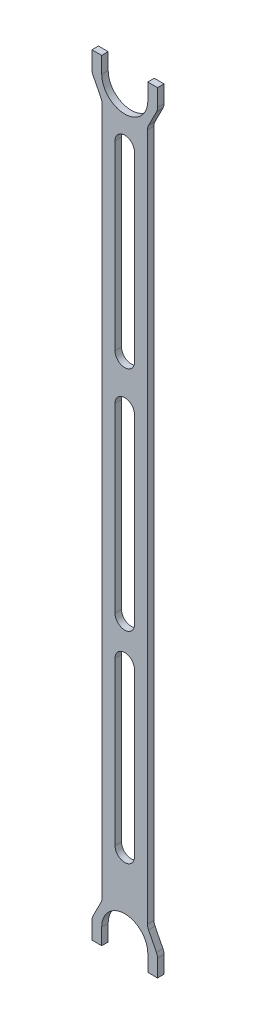
from build123d import *

# Parameters (mm, degrees)
EXTRUDE_1_DEPTH = 2
FILLET_1_R      = 3


with BuildPart() as part:
    # 草图1 → 凸台-拉伸1 (new body)
    with BuildSketch(Plane.XY):
        with BuildLine():
            Line((-7, 106.65), (-7, -106.65))
            Line((-7, -106.65), (-10.1, -112.75))
            Line((-10.1, -112.75), (-10.1, -118.75))
            Line((-10.1, -118.75), (-7.1, -118.75))
            Line((-7.1, -118.75), (-7.1, -113.75))
            ThreePointArc((-7.1, -113.75), (0, -106.65), (7.1, -113.75))
            Line((7.1, -113.75), (7.1, -118.75))
            Line((7.1, -118.75), (10.1, -118.75))
            Line((10.1, -118.75), (10.1, -112.75))
            Line((10.1, -112.75), (7, -106.65))
            Line((7, -106.65), (7, 106.65))
            Line((7, 106.65), (10.1, 112.75))
            Line((10.1, 112.75), (10.1, 118.75))
            Line((10.1, 118.75), (7.1, 118.75))
            Line((7.1, 118.75), (7.1, 113.75))
            ThreePointArc((7.1, 113.75), (0, 106.65), (-7.1, 113.75))
            Line((-7.1, 113.75), (-7.1, 118.75))
            Line((-7.1, 118.75), (-10.1, 118.75))
            Line((-10.1, 118.75), (-10.1, 112.75))
            Line((-10.1, 112.75), (-7, 106.65))
        make_face()
        with BuildLine():
            Line((3, 98), (3, 42))
            ThreePointArc((3, 42), (0, 39), (-3, 42))
            Line((-3, 42), (-3, 98))
            ThreePointArc((-3, 98), (0, 101), (3, 98))
        make_face(mode=Mode.SUBTRACT)
        with BuildLine():
            Line((3, 28), (3, -28))
            ThreePointArc((3, -28), (0, -31), (-3, -28))
            Line((-3, -28), (-3, 28))
            ThreePointArc((-3, 28), (0, 31), (3, 28))
        make_face(mode=Mode.SUBTRACT)
        with BuildLine():
            Line((3, -40), (3, -90))
            ThreePointArc((3, -90), (0, -93), (-3, -90))
            Line((-3, -90), (-3, -40))
            ThreePointArc((-3, -40), (0, -37), (3, -40))
        make_face(mode=Mode.SUBTRACT)
    extrude(amount=EXTRUDE_1_DEPTH)

    # 圆角1
    fillet_1_edges = [part.edges().sort_by_distance(p)[0] for p in [
        (10.1, 112.75, 1),
        (7, 106.65, 1),
        (7, -106.65, 1),
        (10.1, -112.75, 1),
        (-10.1, -112.75, 1),
        (-7, -106.65, 1),
        (-7, 106.65, 1),
        (-10.1, 112.75, 1),
    ]]
    fillet(fillet_1_edges, radius=FILLET_1_R)


solid = part.part
